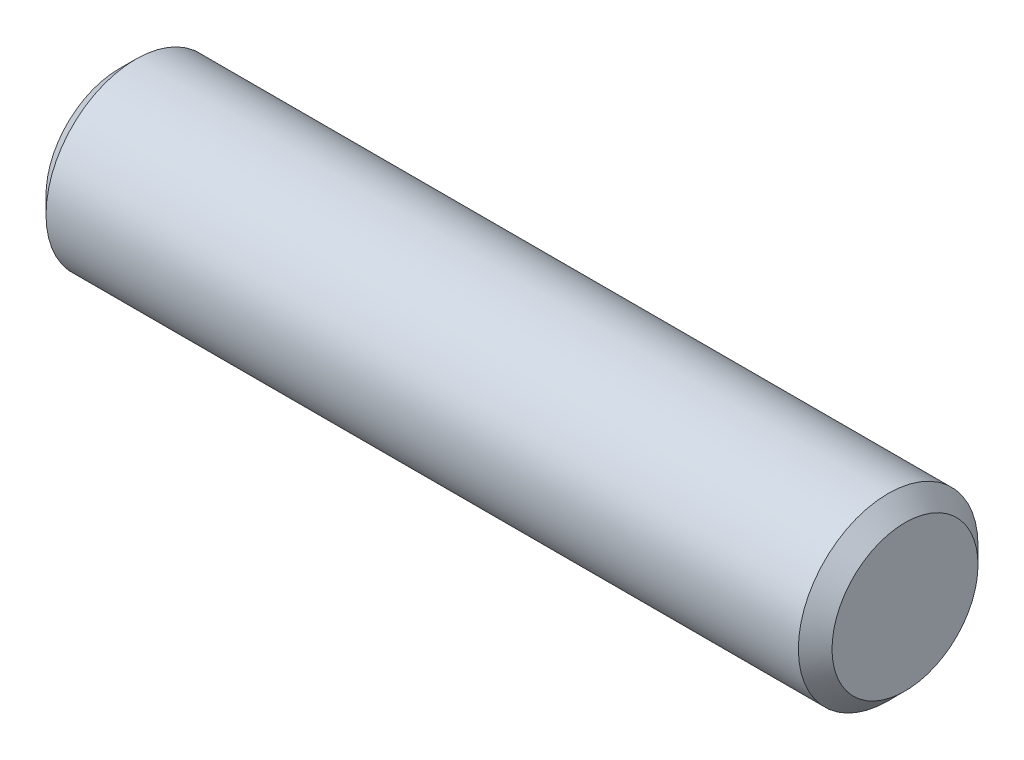
from build123d import *


with BuildPart() as part:
    # Sketch1 → Revolve1 (revolve)
    with BuildSketch(Plane.XY):
        Polygon((-70, 14.5), (-70, 8), (0, 8), (0, 14.5), (-1.5, 16), (-68.5, 16), align=None)
    revolve(axis=Axis((-70, 8, 0), (1, 0, 0)))


solid = part.part
